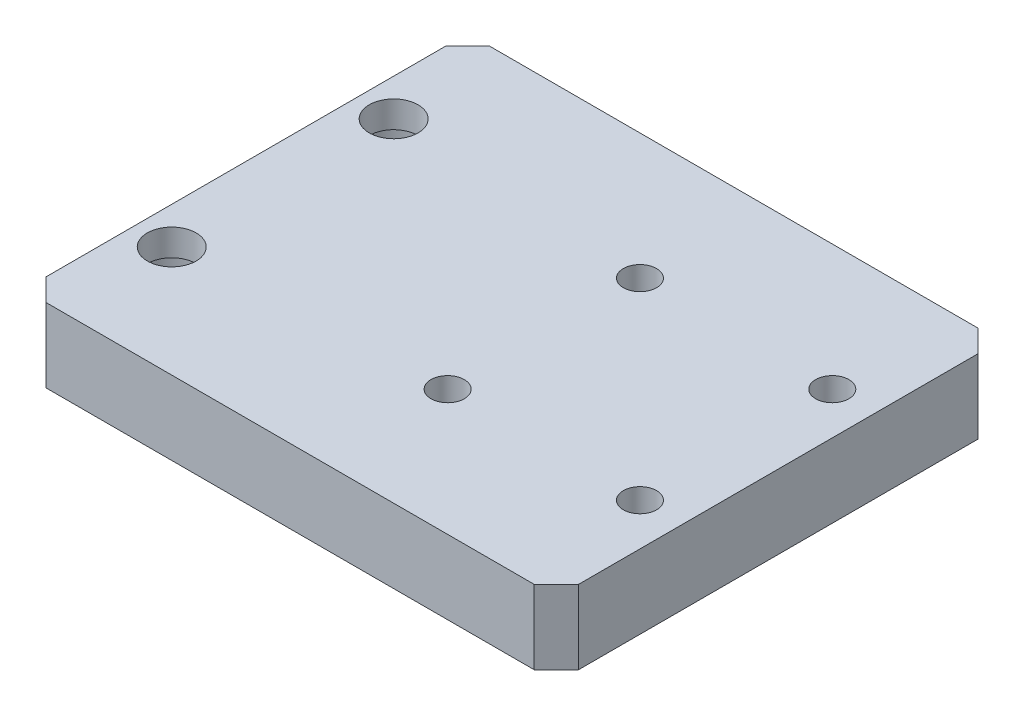
SolidWorks part; units mm, degrees
material "6061-T6"
ref_plane "前视基准面" through (0, 0, 0) normal (0, 0, 1) x (1, 0, 0)
ref_plane "上视基准面" through (0, 0, 0) normal (0, 1, 0) x (1, 0, 0)
ref_plane "右视基准面" through (0, 0, 0) normal (1, 0, 0) x (0, 0, -1)
sketch "草图2" plane through (0, 0, 0) normal (0, 0, 1) x (1, 0, 0)
  line L0 (0, 0) -> (0, -54)
  line L1 (0, -54) -> (72, -54)
  line L2 (10, 0) -> (10, -44)
  line L3 (10, -44) -> (72, -44)
  line L4 (0, 0) -> (10, 0)
  line L5 (72, -54) -> (72, -44)
  dimension "D1" = 72
  dimension "D2" = 54
  dimension "D3" = 10
extrude "凸台-拉伸1" add sketch "草图2" along normal blind 60
hole_wizard "M6 螺纹孔2" positions "草图3" profile "草图4" tap size "M6" standard "ISO"
sketch "草图3" plane through (0, 0, 0) normal (0, 0, -1) x (-1, 0, 0)
  line L0 (-60, -49) -> (-72, -49) construction
  line L1 (-72, -54) -> (-72, -44) construction
  point P0 (-60, -49)
  dimension "D1" = 12
sketch "草图4" plane through (60, -49, 0) normal (1, 0, 0) x (0, 1, 0)
  line L0 (0, 0) -> (0, 18.5022)
  line L1 (0, 18.5022) -> (2.5, 17)
  line L2 (2.5, 17) -> (2.5, 0)
  line L5 (2.5, 0) -> (0, 0)
  line L10 (0, 18.5022) -> (-2.5, 17) construction
  line L11 (0, -6.35) -> (0, 107.95) construction
  dimension "螺纹孔钻头直径" = 5
  dimension "螺纹孔钻头深度" = 17
  dimension "导头角度" = 118
cosmetic thread "孔螺蚊线1" parameters "D1"=12, "D2"=6
hole_wizard "M4 六角凹头螺钉的柱形沉头孔1" positions "草图5" profile "草图6" counterbore size "M4" standard "ISO"
sketch "草图5" plane through (0, -54, 0) normal (0, -1, 0) x (-1, 0, 0)
  point P0 (-40.3, -17)
  point P2 (-66.3, -17)
  point P4 (-66.3, -43)
  point P6 (-40.3, -43)
sketch "草图6" plane through (40.3, -54, 17) normal (1, 0, 0) x (0, 0, -1)
  line L0 (0, 0) -> (0, 12.8519)
  line L1 (0, 12.8519) -> (2.25, 11.5)
  line L2 (2.25, 11.5) -> (2.25, 4.4)
  line L3 (2.25, 4.4) -> (4, 4.4)
  line L4 (4, 4.4) -> (4, 0)
  line L5 (4, 0) -> (0, 0)
  line L10 (0, 12.8519) -> (-2.25, 11.5) construction
  line L11 (0, -6.35) -> (0, 107.95) construction
  dimension "孔直径" = 4.5
  dimension "孔深度" = 11.5
  dimension "柱形沉头孔直径" = 8
  dimension "柱形沉头孔深度" = 4.4
  dimension "导头角度" = 118
hole_wizard "M6 螺纹孔1" positions "草图7" profile "草图8" tap size "M6" standard "ISO"
sketch "草图7" plane through (0, 0, 0) normal (0, 1, 0) x (1, 0, 0)
  point P0 (5, -15)
  point P2 (5, -45)
sketch "草图8" plane through (5, 0, 15) normal (1, 0, 0) x (0, 0, 1)
  line L0 (0, 0) -> (0, 18.5022)
  line L1 (0, 18.5022) -> (2.5, 17)
  line L2 (2.5, 17) -> (2.5, 0)
  line L5 (2.5, 0) -> (0, 0)
  line L10 (0, 18.5022) -> (-2.5, 17) construction
  line L11 (0, -6.35) -> (0, 107.95) construction
  dimension "螺纹孔钻头直径" = 5
  dimension "螺纹孔钻头深度" = 17
  dimension "导头角度" = 118
cosmetic thread "孔螺蚊线2" parameters "D1"=12, "D2"=6
cosmetic thread "孔螺蚊线3" parameters "D1"=12, "D2"=6
chamfer "倒角1" distance 3 angle 45 4 edges at (72, -49, 60) (72, -49, 0) (5, 0, 0) (5, 0, 60)
sketch "草图9" plane through (0, 0, 60) normal (0, 0, 1) x (1, 0, 0)
  line L1 (10, -44) -> (0, -44)
  line L2 (10, -44) -> (10, 0)
  line L3 (10, 0) -> (0, 0)
  line L4 (0, -44) -> (0, 0)
extrude "切除-拉伸1" cut sketch "草图9" against normal through all
chamfer "倒角2" distance 3 angle 45 2 edges at (0, -49, 0) (0, -49, 60)
hole_wizard "M6 六角凹头螺钉的柱形沉头孔1" positions "草图10" profile "草图11" counterbore size "M6" standard "ISO"
sketch "草图10" plane through (0, -54, 0) normal (0, -1, 0) x (-1, 0, 0)
  line L0 (-5, -45) -> (-5, -15) construction
  line L3 (-5, -30) -> (0, -30) construction
  line L4 (0, -57) -> (0, -3) construction
  line L6 (-3, -60) -> (-69, -60) construction
  point P0 (-5, -15)
  point P2 (-5, -45)
  dimension "D1" = 5
  dimension "D2" = 15
sketch "草图11" plane through (5, -54, 15) normal (1, 0, 0) x (0, 0, -1)
  line L0 (0, 0) -> (0, 18.9828)
  line L1 (0, 18.9828) -> (3.3, 17)
  line L2 (3.3, 17) -> (3.3, 6.4)
  line L3 (3.3, 6.4) -> (5.5, 6.4)
  line L4 (5.5, 6.4) -> (5.5, 0)
  line L5 (5.5, 0) -> (0, 0)
  line L10 (0, 18.9828) -> (-3.3, 17) construction
  line L11 (0, -6.35) -> (0, 107.95) construction
  dimension "孔直径" = 6.6
  dimension "孔深度" = 17
  dimension "柱形沉头孔直径" = 11
  dimension "柱形沉头孔深度" = 6.4
  dimension "导头角度" = 118
